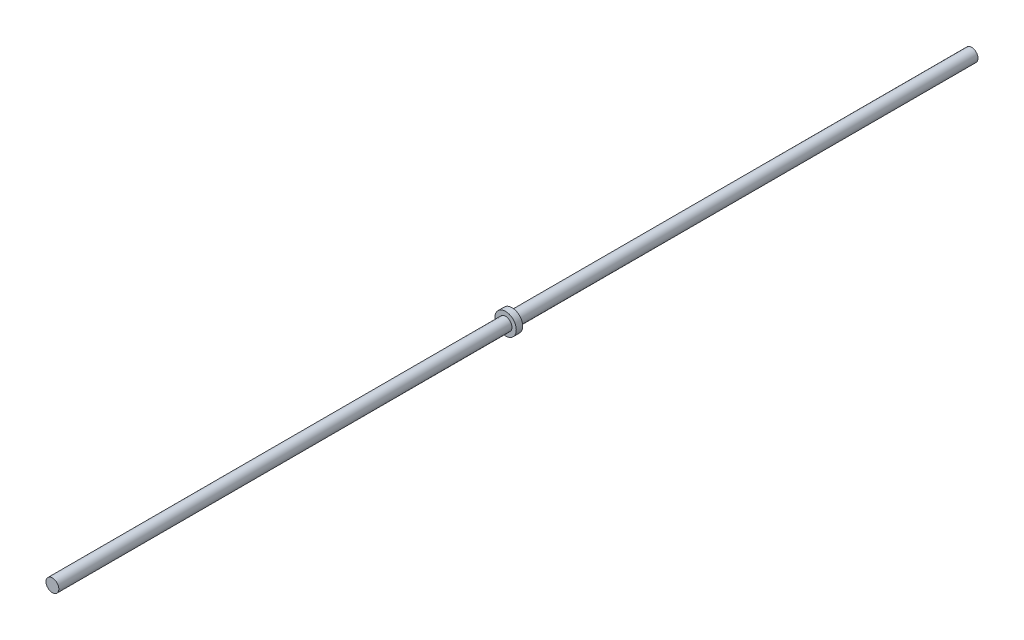
SolidWorks part; units mm, degrees
ref_plane "前视基准面" through (0, 0, 0) normal (0, 0, 1) x (1, 0, 0)
ref_plane "上视基准面" through (0, 0, 0) normal (0, 1, 0) x (1, 0, 0)
ref_plane "右视基准面" through (0, 0, 0) normal (1, 0, 0) x (0, 0, -1)
sketch "草图1" plane through (0, 0, 0) normal (0, 1, 0) x (1, 0, 0)
  line L0 (0, 0) -> (0, 598.1384) construction
  line L1 (0, 0) -> (3, 0)
  line L2 (3, 0) -> (3, 430)
  line L5 (0, 430) -> (0, 0)
  line L6 (3, 430) -> (0, 430)
  dimension "D1" = 430
  dimension "D2" = 3
revolve "旋转1" add sketch "草图1" angle 360 about L0
sketch "草图3" plane through (0, 0, 0) normal (0, 0, 1) x (1, 0, 0)
  circle A0 centre (0, 0) radius 5
  dimension "D1" = 10
extrude "凸台-拉伸1" add sketch "草图3" along normal blind 3 from offset 215
